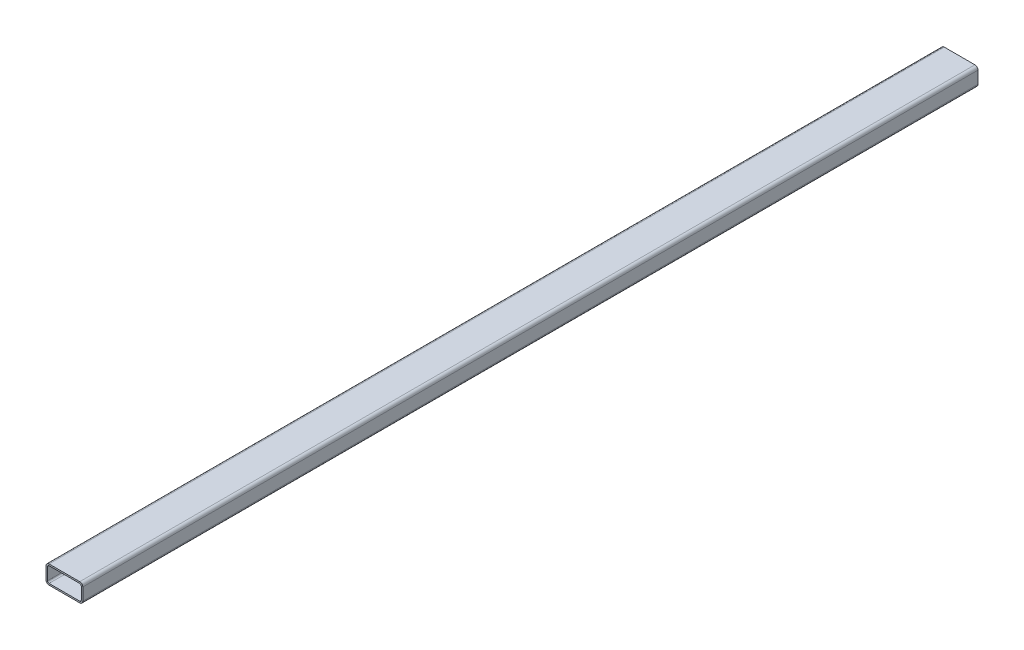
SolidWorks part; units mm, degrees
material "普通碳钢"
ref_plane "Front Plane" through (0, 0, 0) normal (0, 0, 1) x (1, 0, 0)
ref_plane "Top Plane" through (0, 0, 0) normal (0, 1, 0) x (1, 0, 0)
ref_plane "Right Plane" through (0, 0, 0) normal (1, 0, 0) x (0, 0, -1)
sketch "Sketch1" plane through (0, 0, 0) normal (0, 0, 1) x (1, 0, 0)
  line L0 (10, 55) -> (110, 55)
  line L1 (10, 0) -> (110, 0)
  line L2 (0, 10) -> (0, 50)
  line L3 (10, 60) -> (110, 60)
  line L4 (120, 10) -> (120, 50)
  line L5 (115, 10) -> (115, 50)
  line L6 (10, 5) -> (110, 5)
  line L7 (5, 10) -> (5, 50)
  arc A0 (120, 10) -> (110, 0) centre (110, 10) cw
  arc A1 (0, 50) -> (10, 60) centre (10, 50) cw
  arc A2 (120, 50) -> (110, 60) centre (110, 50) ccw
  arc A3 (10, 0) -> (0, 10) centre (10, 10) cw
  arc A4 (115, 50) -> (110, 55) centre (110, 50) ccw
  arc A5 (115, 10) -> (110, 5) centre (110, 10) cw
  arc A6 (10, 5) -> (5, 10) centre (10, 10) cw
  arc A7 (5, 50) -> (10, 55) centre (10, 50) cw
  point P7 (120, 0)
  point P10 (0, 60)
  point P13 (120, 60)
  point P16 (0, 0)
  dimension "D3" = 10
  dimension "D4" = 10
  dimension "D5" = 10
  dimension "D6" = 10
  dimension "D1" = 120
  dimension "D2" = 60
  dimension "D7" = 5
extrude "Boss-Extrude1" add sketch "Sketch1" along normal blind 2920
